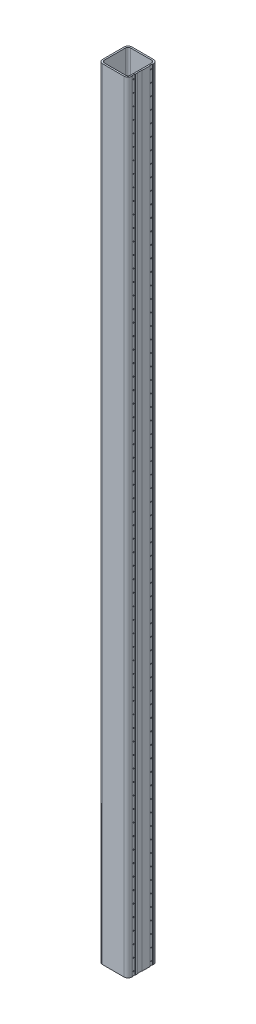
from build123d import *

# Parameters (mm, degrees)
BOSS_EXTRUDE1_DEPTH  = 2000
SKETCH2_W            = 2
SKETCH2_H            = 15
SKETCH2_W_2          = 1.5
SKETCH2_H_2          = 25
CUT_EXTRUDE1_DEPTH   = 4000
CUT_EXTRUDE2_REACH   = 2008.87
SKETCH4_R            = 2.6
LPATTERN2_COUNT      = 2
LPATTERN2_PITCH      = 90.4
LPATTERN2_COUNT_DIR2 = 67
LPATTERN2_PITCH_DIR2 = 60


with BuildPart() as part:
    # Sketch1 → Boss-Extrude1 (new, symmetric)
    with BuildSketch(Plane(origin=(0, 0, 0), x_dir=(1, 0, 0), z_dir=(0, 1, 0))):
        with BuildLine():
            Line((-55, -75), (55, -75))
            ThreePointArc((55, -75), (69.142135624, -69.142135624), (75, -55))
            Line((75, -55), (75, 55))
            ThreePointArc((75, 55), (69.142135624, 69.142135624), (55, 75))
            Line((55, 75), (-55, 75))
            ThreePointArc((-55, 75), (-69.142135624, 69.142135624), (-75, 55))
            Line((-75, 55), (-75, -55))
            ThreePointArc((-75, -55), (-69.142135624, -69.142135624), (-55, -75))
        make_face()
        with BuildLine():
            Line((-67, -55), (-67, 55))
            ThreePointArc((-67, 55), (-63.485281374, 63.485281374), (-55, 67))
            Line((-55, 67), (55, 67))
            ThreePointArc((55, 67), (63.485281374, 63.485281374), (67, 55))
            Line((67, 55), (67, -55))
            ThreePointArc((67, -55), (63.485281374, -63.485281374), (55, -67))
            Line((55, -67), (-55, -67))
            ThreePointArc((-55, -67), (-63.485281374, -63.485281374), (-67, -55))
        make_face(mode=Mode.SUBTRACT)
    extrude(amount=BOSS_EXTRUDE1_DEPTH, both=True)

    # Sketch2 → Cut-Extrude1 (cut)
    with BuildSketch(Plane.XZ.offset(2000)):
        with Locations((74, 45.2)):
            Rectangle(SKETCH2_W, SKETCH2_H)
        with Locations((74, -45.2)):
            Rectangle(SKETCH2_W, SKETCH2_H)
        with Locations((74.25, 14.7)):
            Rectangle(SKETCH2_W_2, SKETCH2_H_2)
    extrude(amount=-CUT_EXTRUDE1_DEPTH, mode=Mode.SUBTRACT)

    # Sketch4 → Cut-Extrude2 (cut, up to next)
    with BuildSketch(Plane(origin=(73, 0, 0), x_dir=(0, 0, -1), z_dir=(1, 0, 0)), mode=Mode.PRIVATE) as cut_extrude2_sk1:
        with Locations((-45.2, -1980)):
            Circle(SKETCH4_R)
    cut_extrude2_tool1 = extrude(cut_extrude2_sk1.sketch, amount=-CUT_EXTRUDE2_REACH, mode=Mode.PRIVATE) & part.part
    cut_extrude2 = cut_extrude2_tool1.solids().sort_by_distance((73, -1980, 45.2))[0]
    add(cut_extrude2, mode=Mode.SUBTRACT)

    # LPattern2: Cut-Extrude2 2 × 67
    with Locations(*[(0, j * LPATTERN2_PITCH_DIR2, -i * LPATTERN2_PITCH) for i in range(LPATTERN2_COUNT) for j in range(LPATTERN2_COUNT_DIR2) if (i, j) != (0, 0)]):
        add(cut_extrude2, mode=Mode.SUBTRACT)


solid = part.part
